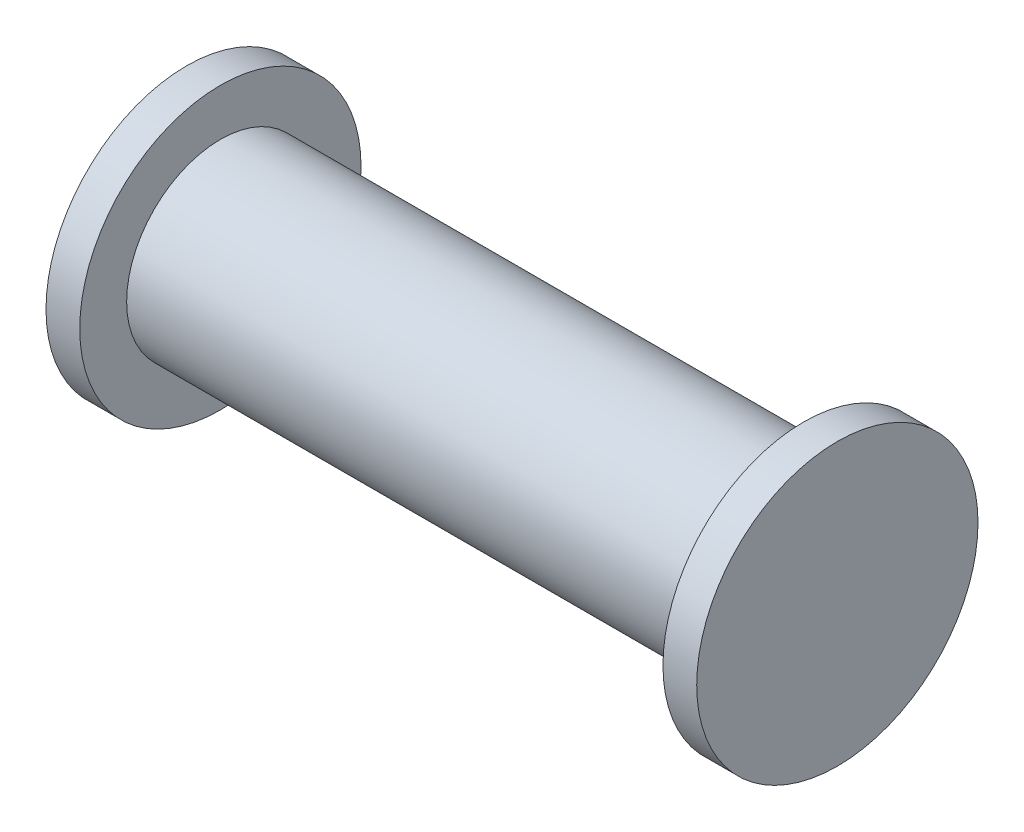
from build123d import *

# Parameters (mm, degrees)
SKETCH_1_4_R        = 75
BOSS_EXTRUDE1_DEPTH = 18
SKETCH_1_3_R        = 50
BOSS_EXTRUDE2_DEPTH = 311
BOSS_EXTRUDE3_START = -329
SKETCH_1_4_2_R      = 75
BOSS_EXTRUDE3_DEPTH = 18


with BuildPart() as part:
    # Sketch 1_4 → Boss-Extrude1 (new body)
    with BuildSketch(Plane(origin=(0, 0, 0), x_dir=(0, 0, -1), z_dir=(1, 0, 0))):
        Circle(SKETCH_1_4_R)
    extrude(amount=BOSS_EXTRUDE1_DEPTH)

    # 草图1<3> → Boss-Extrude2 (add)
    with BuildSketch(Plane(origin=(0, 0, 0), x_dir=(0, 0, -1), z_dir=(1, 0, 0))):
        Circle(SKETCH_1_3_R)
    extrude(amount=-BOSS_EXTRUDE2_DEPTH)

    # Sketch 1_4 2 → Boss-Extrude3 (add)
    with BuildSketch(Plane(origin=(0, 0, 0), x_dir=(0, 0, -1), z_dir=(1, 0, 0)).offset(BOSS_EXTRUDE3_START)):
        Circle(SKETCH_1_4_2_R)
    extrude(amount=BOSS_EXTRUDE3_DEPTH)


solid = part.part
